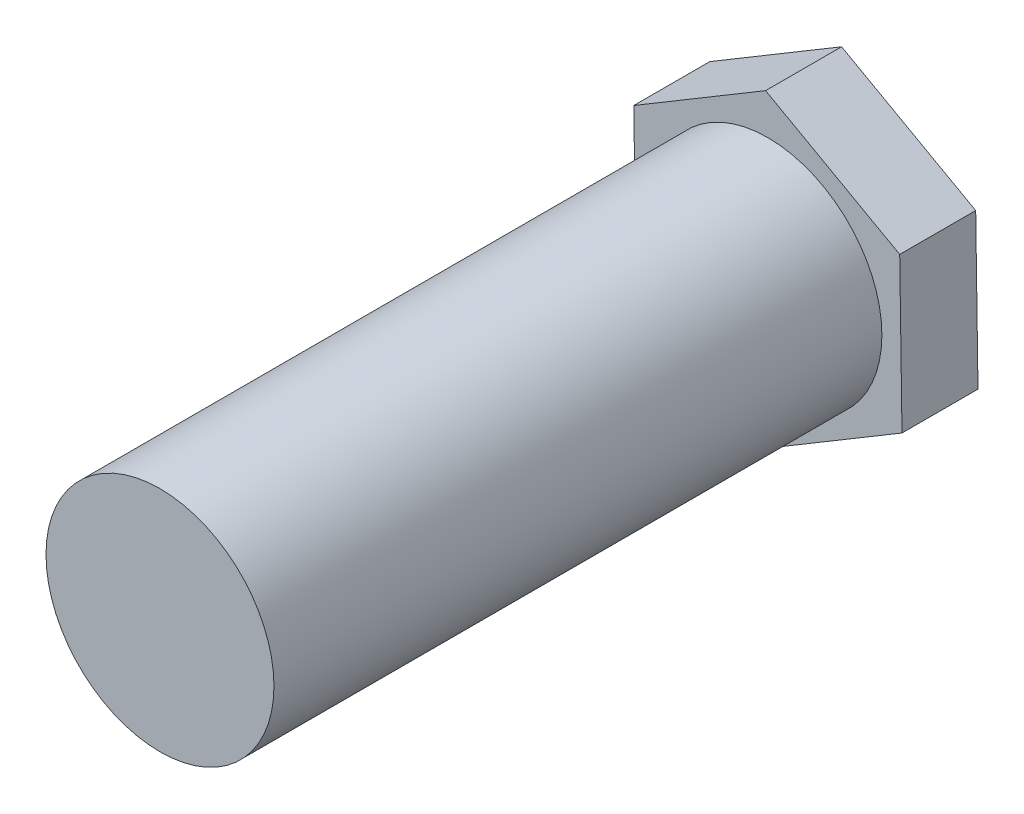
SolidWorks part; units mm, degrees
ref_plane "Front Plane" through (0, 0, 0) normal (0, 0, 1) x (1, 0, 0)
ref_plane "Top Plane" through (0, 0, 0) normal (0, 1, 0) x (1, 0, 0)
ref_plane "Right Plane" through (0, 0, 0) normal (1, 0, 0) x (0, 0, -1)
other "Configuration Table"
sketch "Sketch1" plane through (0, 0, 0) normal (0, 0, 1) x (1, 0, 0)
  line L13 (17.3465, 10.3649) -> (-0.303, 20.205)
  line L14 (-0.303, 20.205) -> (-17.6496, 9.8401)
  line L15 (-17.6496, 9.8401) -> (-17.3465, -10.3649)
  line L16 (-17.3465, -10.3649) -> (0.303, -20.205)
  line L17 (0.303, -20.205) -> (17.6496, -9.8401)
  line L18 (17.6496, -9.8401) -> (17.3465, 10.3649)
  circle A1 centre (0, 0) radius 17.5 construction
  dimension "D1" = 35
extrude "Boss-Extrude1" add sketch "Sketch1" along normal blind 10
sketch "Sketch2" plane through (0, 0, 10) normal (0, 0, 1) x (1, 0, 0)
  circle A0 centre (0, 0) radius 15
  dimension "D1" = 30
extrude "Boss-Extrude2" add sketch "Sketch2" along normal blind 80
cosmetic thread "Cosmetic Thread1" parameters "D2"=26.211
cosmetic thread "Cosmetic Thread2" parameters "D2"=26.211
